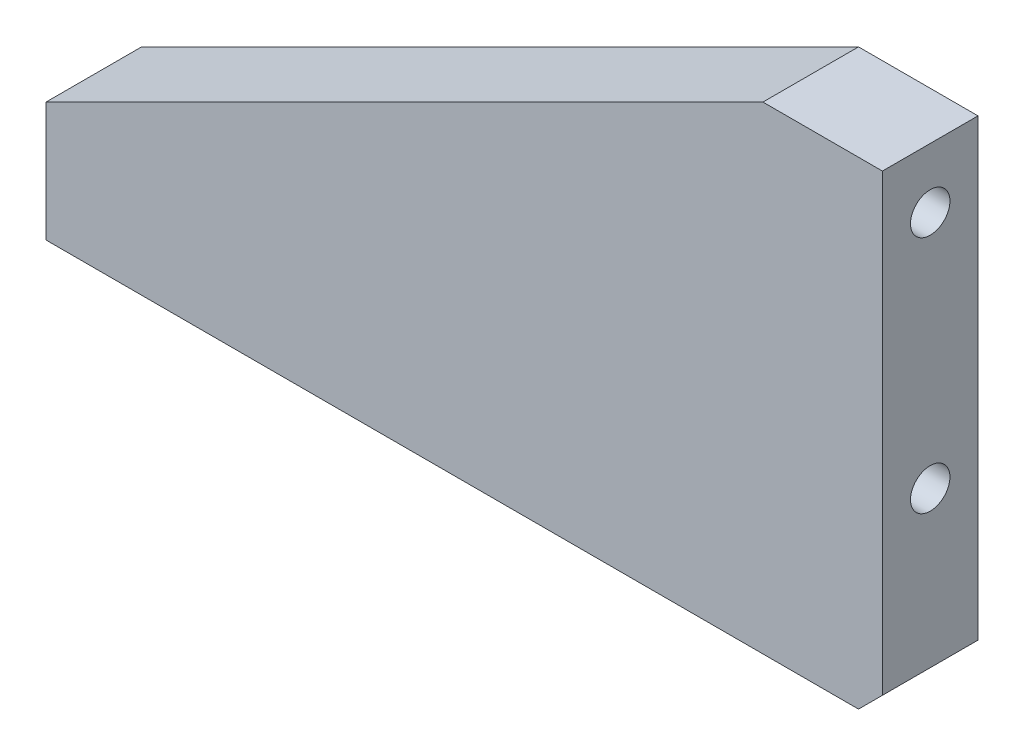
from build123d import *

# Parameters (mm, degrees)
EXTRUDE_1_DEPTH        = 8
HOLE_WIZARD_M4_2_D     = 3.3
HOLE_WIZARD_M4_2_DEPTH = 10.1
HOLE_WIZARD_M4_2_TIP   = 0.991420021
HOLE_WIZARD_M4_1_D     = 3.3
HOLE_WIZARD_M4_1_DEPTH = 10.1
HOLE_WIZARD_M4_1_TIP   = 0.991420021
CHAMFER_1_SIZE         = 2


with BuildPart() as part:
    # 草图1 → 凸台-拉伸1 (new body)
    with BuildSketch(Plane.XY):
        Polygon((0, 0), (0, 40), (-10, 40), (-70, 10), (-70, 0), align=None)
    extrude(amount=EXTRUDE_1_DEPTH)

    # M4 螺纹孔2
    with Locations(Plane(origin=(0, 0, 0), x_dir=(-1, 0, 0), z_dir=(0, -1, 0))):
        with Locations((15, -4), (65, -4)):
            Hole(HOLE_WIZARD_M4_2_D / 2, depth=HOLE_WIZARD_M4_2_DEPTH)
            with Locations((0, 0, -(HOLE_WIZARD_M4_2_DEPTH + HOLE_WIZARD_M4_2_TIP / 2))):  # 118° drill point
                Cone(0, HOLE_WIZARD_M4_2_D / 2, HOLE_WIZARD_M4_2_TIP, mode=Mode.SUBTRACT)

    # M4 螺纹孔1
    with Locations(Plane(origin=(0, 0, 0), x_dir=(0, 0, -1), z_dir=(1, 0, 0))):
        with Locations((-4, 35), (-4, 15)):
            Hole(HOLE_WIZARD_M4_1_D / 2, depth=HOLE_WIZARD_M4_1_DEPTH)
            with Locations((0, 0, -(HOLE_WIZARD_M4_1_DEPTH + HOLE_WIZARD_M4_1_TIP / 2))):  # 118° drill point
                Cone(0, HOLE_WIZARD_M4_1_D / 2, HOLE_WIZARD_M4_1_TIP, mode=Mode.SUBTRACT)

    # 倒角1
    chamfer_1_edges = [part.edges().sort_by_distance(p)[0] for p in [
        (0, 0, 4),
    ]]
    chamfer(chamfer_1_edges, length=CHAMFER_1_SIZE)


solid = part.part
